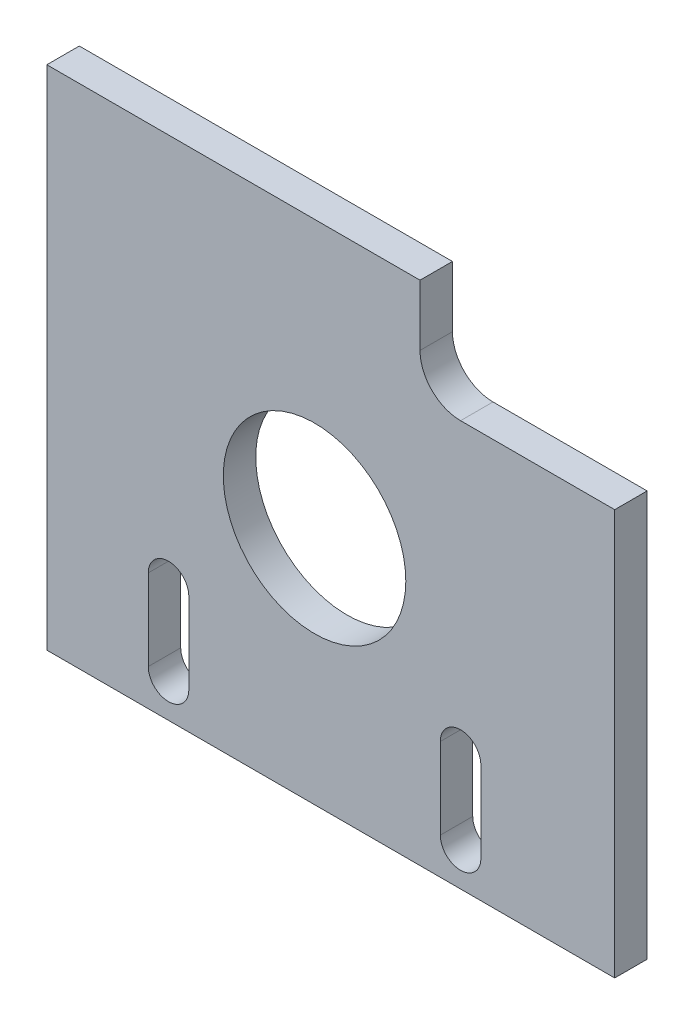
SolidWorks part; units mm, degrees
material "Plain Carbon Steel"
ref_plane "Front Plane" through (0, 0, 0) normal (0, 0, 1) x (1, 0, 0)
ref_plane "Top Plane" through (0, 0, 0) normal (0, 1, 0) x (1, 0, 0)
ref_plane "Right Plane" through (0, 0, 0) normal (1, 0, 0) x (0, 0, -1)
sketch "Sketch1" plane through (0, 0, 0) normal (0, 0, 1) x (1, 0, 0)
  line L1 (0, 0) -> (140, 0)
  line L2 (0, 0) -> (0, -125)
  line L3 (0, -125) -> (140, -125)
  line L4 (140, 0) -> (140, -125)
  dimension "D1" = 125
  dimension "D2" = 140
extrude "Boss-Extrude1" add sketch "Sketch1" along normal blind 8
sketch "Sketch2" plane through (0, 0, 8) normal (0, 0, 1) x (1, 0, 0)
  line L0 (140, 0) -> (0, 0) construction
  line L1 (0, 0) -> (0, -125) construction
  circle A0 centre (66, -66) radius 22.5
  dimension "D3" = 45
  dimension "D1" = 66
  dimension "D2" = 66
extrude "Cut-Extrude1" cut sketch "Sketch2" against normal blind 8
sketch "Sketch3" plane through (0, 0, 8) normal (0, 0, 1) x (1, 0, 0)
  line L0 (30, -96) -> (30, -116) construction
  line L1 (35, -96) -> (35, -116)
  line L2 (25, -96) -> (25, -116)
  line L3 (140, 0) -> (0, 0) construction
  line L4 (0, 0) -> (0, -125) construction
  arc A0 (35, -96) -> (25, -96) centre (30, -96) ccw
  arc A1 (25, -116) -> (35, -116) centre (30, -116) ccw
  point P2 (30, -106)
  dimension "D3" = 5
  dimension "D1" = 106
  dimension "D2" = 30
  dimension "D4" = 20
extrude "Cut-Extrude2" cut sketch "Sketch3" against normal blind 8
pattern_linear "LPattern1" count 2 spacing 72 along (1, 0, 0) of "Cut-Extrude2"
sketch "Sketch4" plane through (0, 0, 8) normal (0, 0, 1) x (1, 0, 0)
  line L0 (140, 0) -> (0, 0) construction
  line L1 (92, 0) -> (140, 0)
  line L2 (92, 0) -> (92, -25)
  line L3 (92, -25) -> (140, -25)
  line L4 (140, 0) -> (140, -25)
  line L5 (140, -125) -> (140, 0) construction
  line L6 (0, 0) -> (0, -125) construction
  dimension "D1" = 25
  dimension "D2" = 92
extrude "Cut-Extrude3" cut sketch "Sketch4" against normal blind 8
fillet "Fillet1" radius 10 1 edges at (92, -25, 4)
